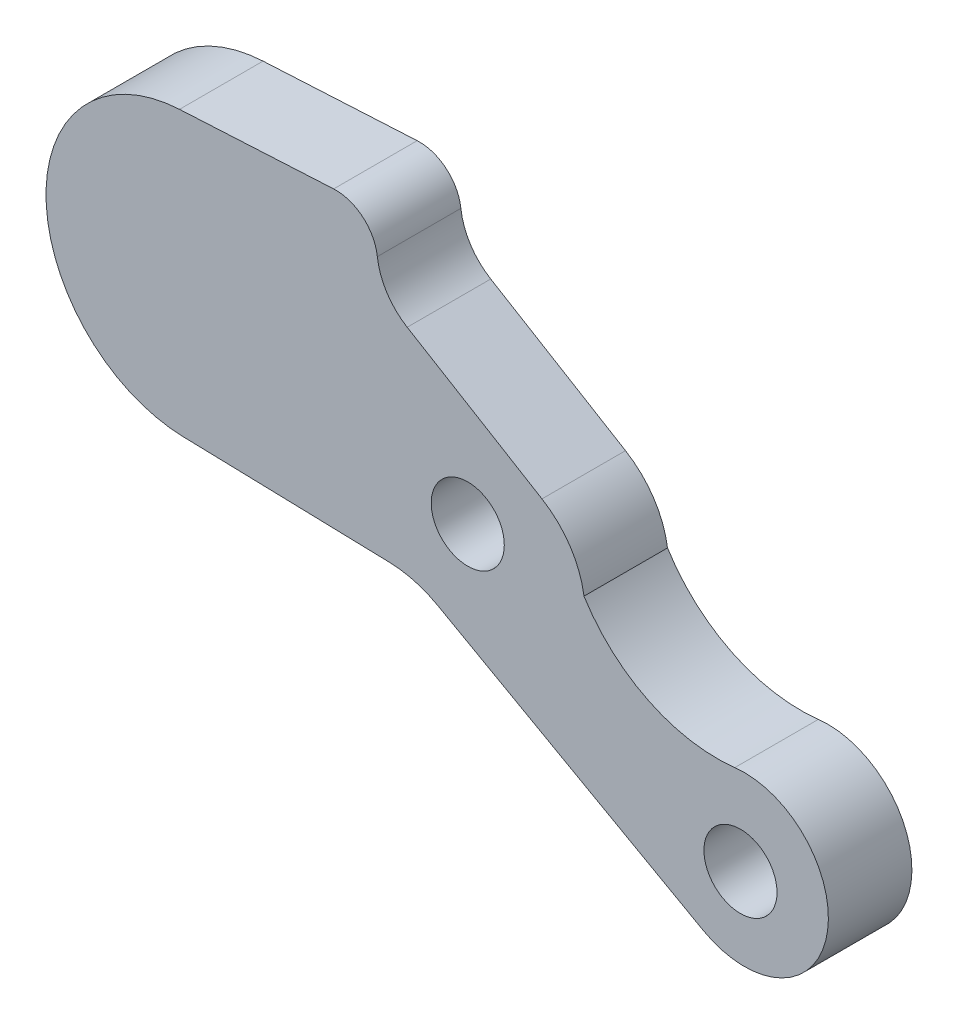
from build123d import *

# Parameters (mm, degrees)
SKETCH1_R           = 3.5
BOSS_EXTRUDE1_DEPTH = 8


with BuildPart() as part:
    # Sketch1 → Boss-Extrude1 (new body)
    with BuildSketch(Plane.XY):
        with BuildLine():
            Line((-5.798172106, 13.421777583), (7.10907715, 5.639148423))
            ThreePointArc((7.10907715, 5.639148423), (9.80078667, 3.06238877), (11.131712033, -0.418075011))
            ThreePointArc((11.131712033, -0.418075011), (17.340118207, -6.010126453), (25.57704331, -7.41312731))
            ThreePointArc((25.57704331, -7.41312731), (34.379390092, -16.99617332), (22.557253019, -22.432454651))
            Line((22.557253019, -22.432454651), (-2.875002754, -8.194359513))
            ThreePointArc((-2.875002754, -8.194359513), (-5.104195022, -7.279113116), (-7.487609197, -6.923710526))
            Line((-7.487609197, -6.923710526), (-27.257727584, -6.38499079))
            ThreePointArc((-27.257727584, -6.38499079), (-40.388886249, 6.936592853), (-27.604263246, 20.591091499))
            Line((-27.604263246, 20.591091499), (-12.841633554, 21.373253968))
            ThreePointArc((-12.841633554, 21.373253968), (-10.053936254, 20.438904782), (-8.658, 17.851313892))
            ThreePointArc((-8.658, 17.851313892), (-7.740710394, 15.305581662), (-5.798172106, 13.421777583))
        make_face()
        Circle(SKETCH1_R, mode=Mode.SUBTRACT)
        with Locations((26.118895321, -15.749708163)):
            Circle(SKETCH1_R, mode=Mode.SUBTRACT)
    extrude(amount=BOSS_EXTRUDE1_DEPTH)


solid = part.part
